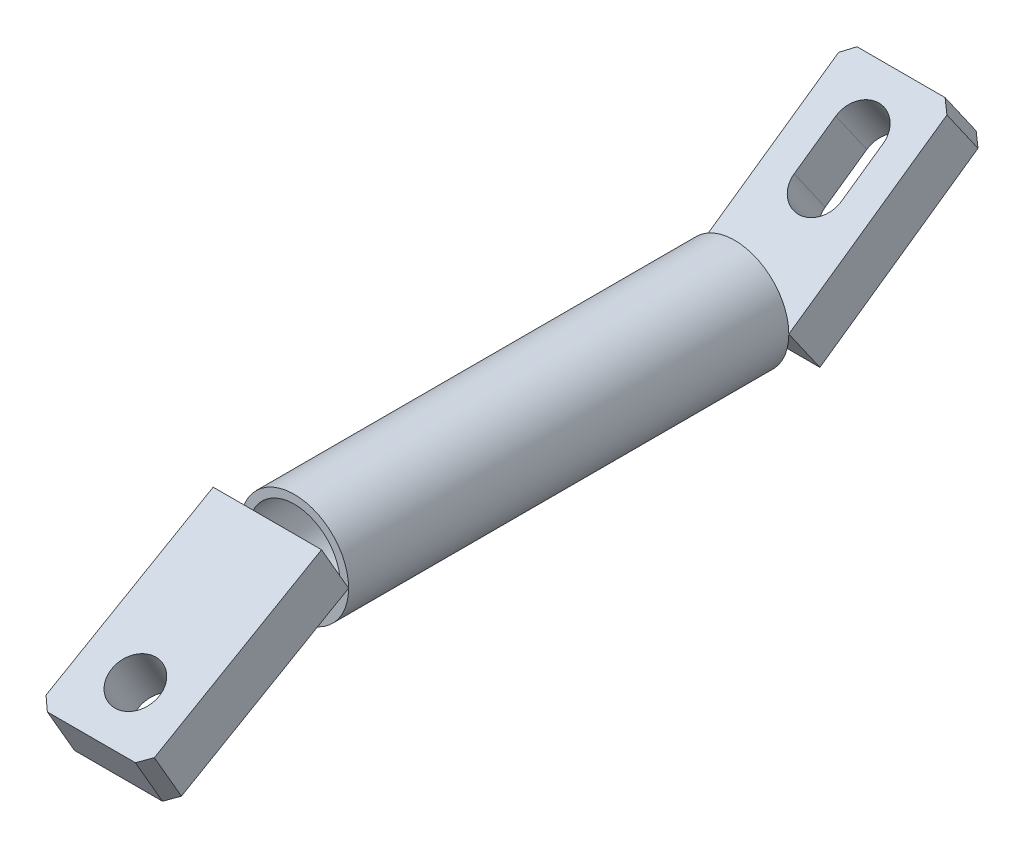
SolidWorks part; units mm, degrees
material "Q235-A "
ref_plane "前视基准面" through (0, 0, 0) normal (0, 0, 1) x (1, 0, 0)
ref_plane "上视基准面" through (0, 0, 0) normal (0, 1, 0) x (1, 0, 0)
ref_plane "右视基准面" through (0, 0, 0) normal (1, 0, 0) x (0, 0, -1)
sketch "草图1" plane through (0, 0, 0) normal (0, 0, 1) x (1, 0, 0)
  circle A0 centre (0, 0) radius 16
  circle A1 centre (0, 0) radius 13.5
  dimension "D1" = 32
  dimension "D2" = 2.5
extrude "凸台-拉伸1" add sketch "草图1" along normal blind 130
sketch "草图2" plane through (0, 0, 0) normal (1, 0, 0) x (0, 0, -1)
  line L0 (4.5886, -6.5532) -> (53.7377, 27.8614) construction
  line L1 (0, 0) -> (49.1491, 34.4146)
  line L2 (0, -16) -> (0, 16) construction
  line L3 (49.1491, 34.4146) -> (58.3263, 21.3082)
  line L4 (58.3263, 21.3082) -> (9.1772, -13.1064)
  line L5 (9.1772, -13.1064) -> (0, 0)
  dimension "D1" = 16
  dimension "D2" = 35
  dimension "D3" = 60
extrude "凸台-拉伸2" add sketch "草图2" along normal mid plane 32 separate body
sketch "草图3" plane through (0, 0, 0) normal (0, 0.8192, 0.5736) x (1, 0, 0)
  line L0 (0, 60) -> (0, 9.1772) construction
  line L1 (16, 60) -> (-16, 60) construction
  line L2 (0, 45) -> (0, 30) construction
  line L3 (7, 45) -> (7, 30)
  line L4 (-7, 45) -> (-7, 30)
  circle A0 centre (0, 45) radius 7 construction
  arc A1 (7, 45) -> (-7, 45) centre (0, 45) ccw
  arc A2 (-7, 30) -> (7, 30) centre (0, 30) ccw
  ellipse E0 centre (0, 0) end of major axis (-16, 0) minor radius 9.1772 construction
  point P13 (0, 37.5)
  dimension "D1" = 14
  dimension "D2" = 15
  dimension "D4" = 7
  dimension "D3" = 15
extrude "切除-拉伸1" cut sketch "草图3" against normal through all
ref_plane "基准面1" through (0, 0, 65) normal (0, 0, 1) x (1, 0, 0)
sketch "草图4" plane through (0, 0, 0) normal (1, 0, 0) x (0, 0, -1)
  line L0 (-130, 16) -> (-130, -16) construction
  line L2 (-189.9615, -16.1436) -> (-181.9615, -30)
  line L3 (-181.9615, -30) -> (-130, 0)
  line L4 (-189.9615, -16.1436) -> (-138, 13.8564)
  line L5 (-138, 13.8564) -> (-130, 0)
  line L6 (-185.9615, -23.0718) -> (-134, 6.9282) construction
  dimension "D1" = 16
  dimension "D2" = 60
  dimension "D3" = 30
extrude "凸台-拉伸3" add sketch "草图4" along normal mid plane 32 separate body
sketch "草图5" plane through (0, 56.2917, 32.5) normal (0, -0.866, -0.5) x (1, 0, 0)
  line L0 (0, 172.5833) -> (0, 157.5833) construction
  line L1 (16, 172.5833) -> (-16, 172.5833) construction
  circle A0 centre (0, 157.5833) radius 7
  dimension "D1" = 14
  dimension "D2" = 15
extrude "切除-拉伸2" cut sketch "草图5" against normal through all
chamfer "倒角1" distance 3 angle 45 2 edges at (16, -23.0718, 185.9615) (-16, -23.0718, 185.9615)
chamfer "倒角2" distance 3 angle 45 2 edges at (16, 27.8614, -53.7377) (-16, 27.8614, -53.7377)
